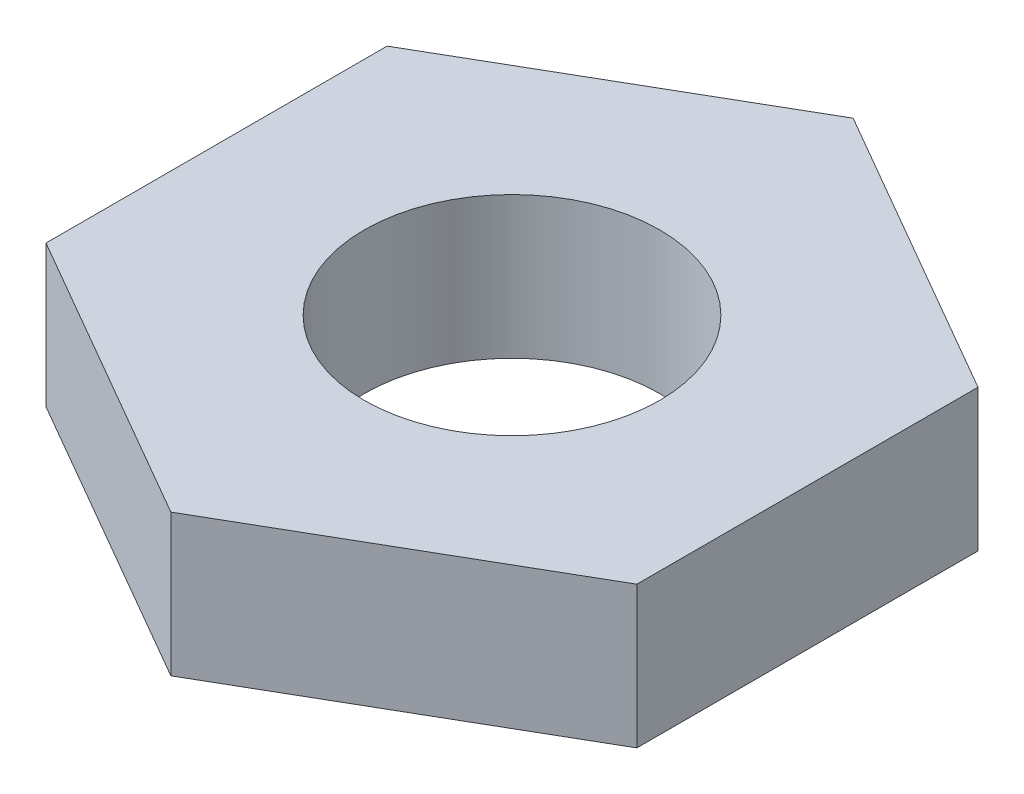
SolidWorks part; units mm, degrees
ref_plane "前视基准面" through (0, 0, 0) normal (0, 0, 1) x (1, 0, 0)
ref_plane "上视基准面" through (0, 0, 0) normal (0, 1, 0) x (1, 0, 0)
ref_plane "右视基准面" through (0, 0, 0) normal (1, 0, 0) x (0, 0, -1)
sketch "草图1" plane through (0, 0, 0) normal (0, 1, 0) x (1, 0, 0)
  line L0 (0, 0) -> (0, 11.4856) construction
  line L1 (0, 5.7735) -> (-5, 2.8868)
  line L2 (-5, 2.8868) -> (-5, -2.8868)
  line L3 (-5, -2.8868) -> (0, -5.7735)
  line L4 (0, -5.7735) -> (5, -2.8868)
  line L5 (5, -2.8868) -> (5, 2.8868)
  line L6 (5, 2.8868) -> (0, 5.7735)
  circle A0 centre (0, 0) radius 5 construction
  dimension "D1" = 10
extrude "凸台-拉伸1" add sketch "草图1" along normal blind 2.4
hole_wizard "M6 螺纹孔1" positions "草图3" profile "草图2" tap size "M6" standard "ISO" end condition through all
sketch "草图3" plane through (0, 2.4, 0) normal (0, 1, 0) x (1, 0, 0)
  point P0 (0, 0)
sketch "草图2" plane through (0, 2.4, 0) normal (1, 0, 0) x (0, 0, 1)
  line L0 (0, 0) -> (0, 2.4)
  line L1 (0, 2.4) -> (2.5, 2.4)
  line L2 (2.5, 2.4) -> (2.5, 0)
  line L5 (2.5, 0) -> (0, 0)
  line L11 (0, -6.35) -> (0, 107.95) construction
  dimension "通孔螺纹孔钻头直径" = 5
  dimension "通孔螺纹孔钻头深度" = 2.4
cosmetic thread "孔螺蚊线1" parameters "D2"=6
